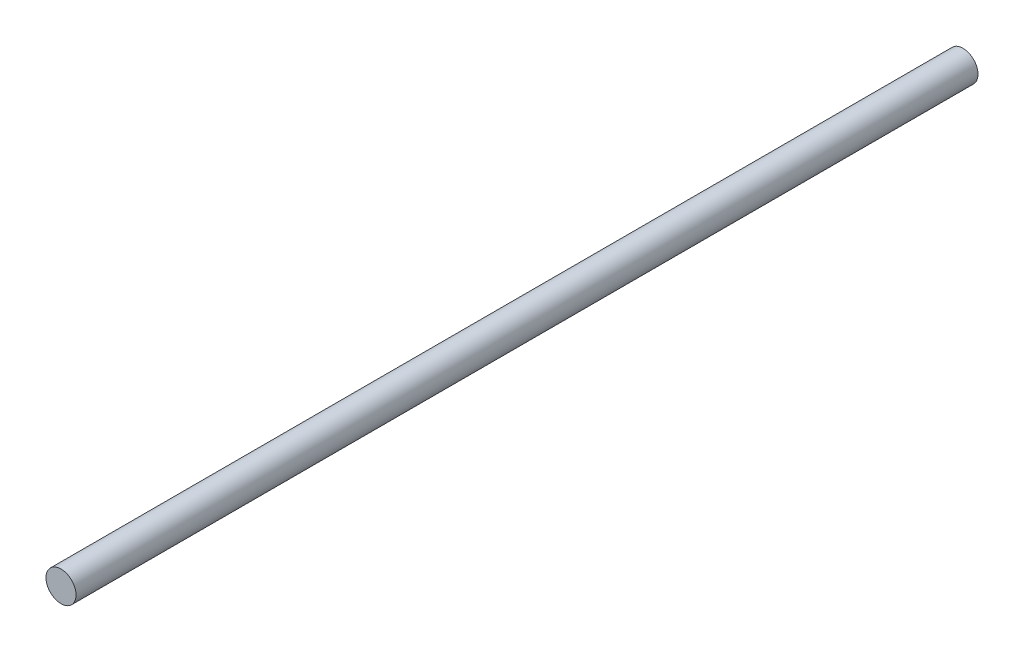
SolidWorks part; units mm, degrees
ref_plane "前视基准面" through (0, 0, 0) normal (0, 0, 1) x (1, 0, 0)
ref_plane "上视基准面" through (0, 0, 0) normal (0, 1, 0) x (1, 0, 0)
ref_plane "右视基准面" through (0, 0, 0) normal (1, 0, 0) x (0, 0, -1)
sketch "草图1" plane through (0, 0, 0) normal (0, 0, 1) x (1, 0, 0)
  circle A0 centre (0, 0) radius 10
  dimension "D1" = 20
extrude "凸台-拉伸1" add sketch "草图1" along normal mid plane 600
